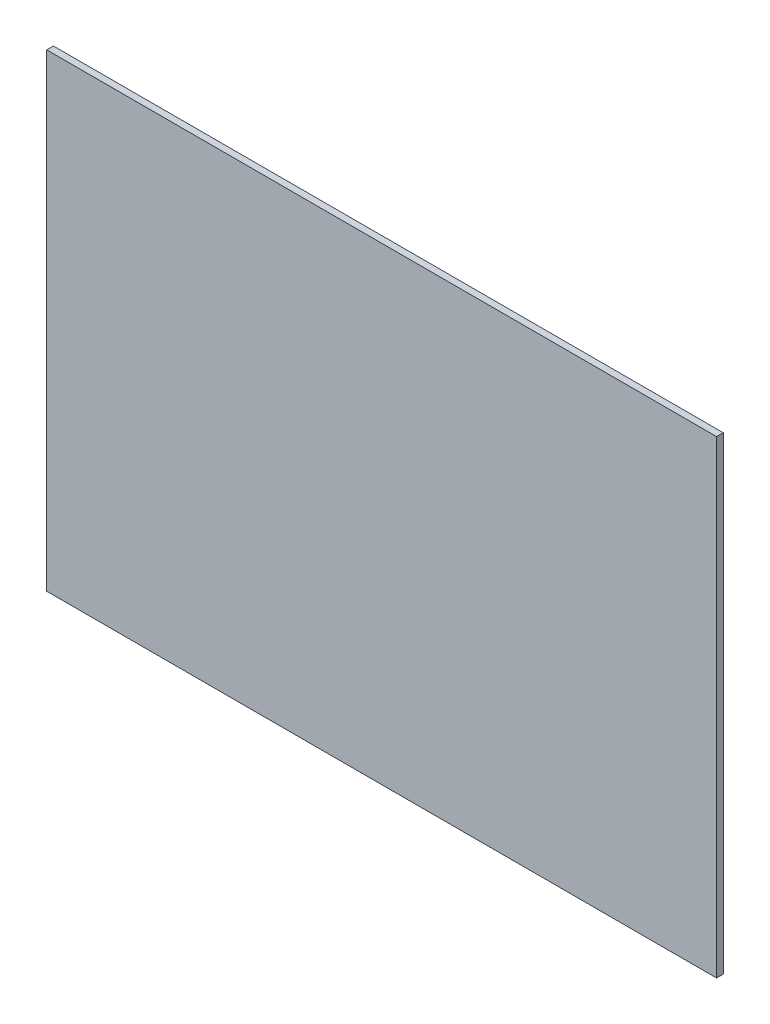
SolidWorks part; units mm, degrees
ref_plane "Front Plane" through (0, 0, 0) normal (0, 0, 1) x (1, 0, 0)
ref_plane "Top Plane" through (0, 0, 0) normal (0, 1, 0) x (1, 0, 0)
ref_plane "Right Plane" through (0, 0, 0) normal (1, 0, 0) x (0, 0, -1)
sketch "Sketch1" plane through (0, 0, 0) normal (0, 0, 1) x (1, 0, 0)
  line L1 (-500, 350) -> (500, 350)
  line L2 (-500, 350) -> (-500, -350)
  line L3 (-500, -350) -> (500, -350)
  line L4 (500, 350) -> (500, -350)
  line L5 (-500, 350) -> (500, -350) construction
  line L6 (-500, -350) -> (500, 350) construction
  point P0 (0, 0)
  dimension "D1" = 1000
  dimension "D2" = 700
extrude "Boss-Extrude1" add sketch "Sketch1" along normal blind 10
